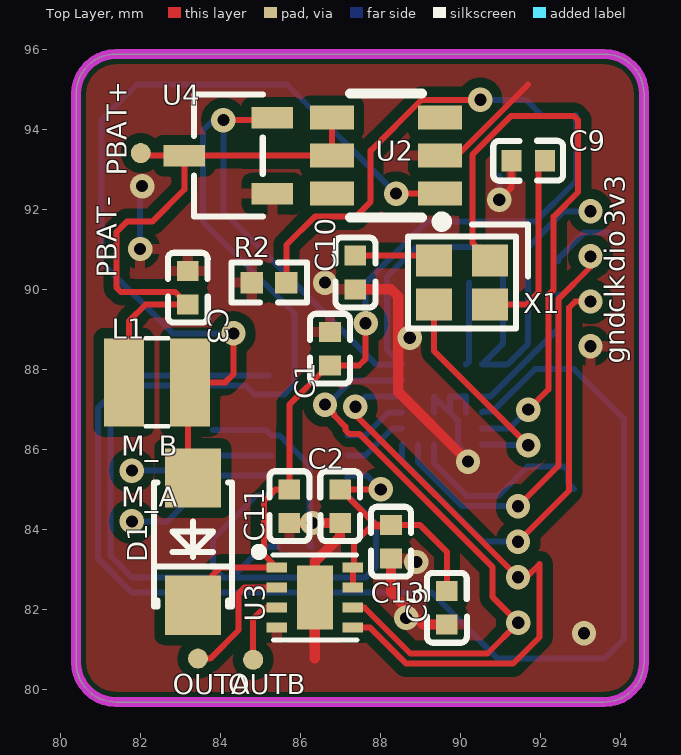
[diagram p0: Top Layer view]
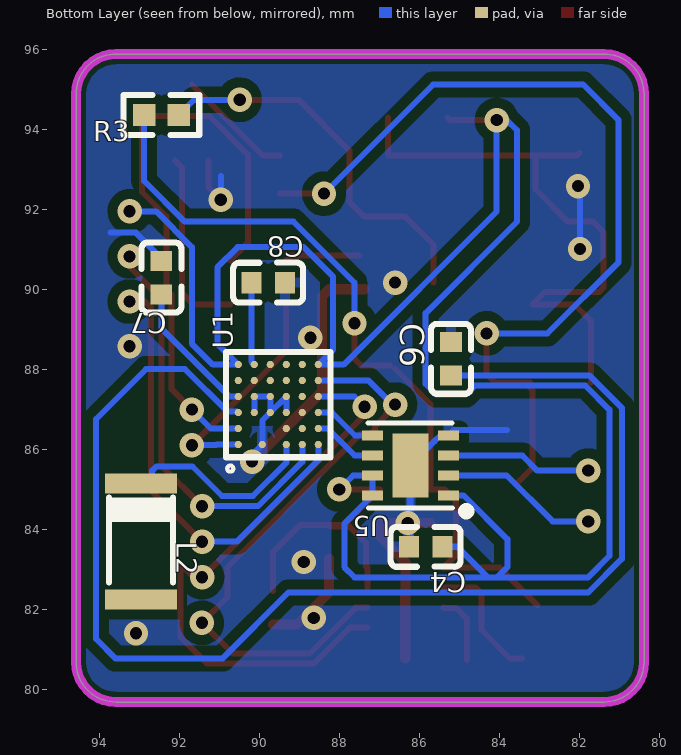
[diagram p1: Bottom Layer view, seen from below]
# Altium PCB MISC49870.pcbdoc
Units mm, origin at the board's own origin, x right, y up, seen from the top; angles counter-clockwise.
Board outline 14.2 x 16.2 mm, 2 copper layers (Top Layer, Bottom Layer), stack 1.58 mm thick; 33 components, 24 nets, 108 pads, 30 vias.

## Layer stack, top to bottom
Top Solder Mask Layer: solder mask 0.01, Dk 3.3
Top Layer: signal copper 0.035
Dielectric1: surface 1.51, FR4, Dk 4.5
Bottom Layer: signal copper 0.035
Bottom Solder Mask Layer: solder mask 0.01, Dk 3.3

## Board outline
81.391,95.885 ccw(c81.391,94.885) 80.391,94.885 80.391,80.685 ccw(c81.391,80.685) 81.391,79.685 93.591,79.685 ccw(c93.591,80.685) 94.591,80.685 94.591,94.885 ccw(c93.591,94.885) 93.591,95.885

## Design rules (kind name [scope] priority, off if disabled: settings)
BoardOutlineClearance copperThickness2oz_1 [All] p2 off: genericclearance=0.203 ignorepadtopadclearanceinfootprint=FALSE except(0: Arc-SplitContinuation Track-SplitContinuation SMDPad-SplitContinuation THPad-SplitContinuation Via-SplitContinuation Fill-SplitContinuation Region-SplitContinuation Poly-SplitContinuation Text-SplitContinuation Hole-SplitContinuation; 0.152: Arc-CutoutEdge SMDPad-CutoutEdge THPad-CutoutEdge Via-CutoutEdge Fill-CutoutEdge Region-CutoutEdge Text-CutoutEdge; 0.176: Hole-OutlineEdge Hole-CutoutEdge; 0.254: Poly-OutlineEdge Poly-CutoutEdge; 0.3: Arc-OutlineEdge Track-OutlineEdge SMDPad-OutlineEdge THPad-OutlineEdge Via-OutlineEdge Fill-OutlineEdge Region-OutlineEdge Text-OutlineEdge Track-CutoutEdge)
BoardOutlineClearance copperThickness1oz_1 [All] p4: genericclearance=0.102 ignorepadtopadclearanceinfootprint=FALSE except(0: Arc-SplitContinuation Track-SplitContinuation SMDPad-SplitContinuation THPad-SplitContinuation Via-SplitContinuation Fill-SplitContinuation Region-SplitContinuation Poly-SplitContinuation Text-SplitContinuation Hole-SplitContinuation; 0.152: SMDPad-CutoutEdge THPad-CutoutEdge Via-CutoutEdge Fill-CutoutEdge Region-CutoutEdge Text-CutoutEdge; 0.176: Hole-OutlineEdge Hole-CutoutEdge; 0.254: Poly-OutlineEdge Poly-CutoutEdge; 0.3: Arc-OutlineEdge Track-OutlineEdge SMDPad-OutlineEdge THPad-OutlineEdge Via-OutlineEdge Fill-OutlineEdge Region-OutlineEdge Text-OutlineEdge Arc-CutoutEdge Track-CutoutEdge)
Clearance copperThickness2oz [All] p1 off: gap=0.203 ignorepadtopadclearanceinfootprint=FALSE except(0.152: SMDPad-Track SMDPad-SMDPad THPad-Track SMDPad-THPad THPad-THPad Track-Via SMDPad-Via THPad-Via Via-Via Fill-Track Region-Track Fill-SMDPad Region-SMDPad Fill-THPad Region-THPad Fill-Via Region-Via Fill-Fill Fill-Region Region-Region Arc-Track Arc-SMDPad Arc-THPad Arc-Via Fill-Arc Region-Arc Arc-Arc Text-Track SMDPad-Text Text-THPad Text-Via Fill-Text Region-Text Arc-Text Text-Text; 0.176: Hole-Track Hole-SMDPad Hole-THPad Hole-Via Fill-Hole Region-Hole Hole-Arc Hole-Text; 0.254: Poly-Track Poly-SMDPad Poly-THPad Poly-Via Poly-Fill Poly-Region Poly-Poly Poly-Arc Poly-Text Poly-Hole)
Clearance copperThickness1oz [All] p3: gap=0.102 ignorepadtopadclearanceinfootprint=FALSE except(0.152: SMDPad-Track SMDPad-SMDPad THPad-Track SMDPad-THPad THPad-THPad Track-Via SMDPad-Via THPad-Via Via-Via Fill-Track Region-Track Fill-SMDPad Region-SMDPad Fill-THPad Region-THPad Fill-Via Region-Via Fill-Fill Fill-Region Region-Region Arc-Track Arc-SMDPad Arc-THPad Arc-Via Fill-Arc Region-Arc Arc-Arc Text-Track SMDPad-Text Text-THPad Text-Via Fill-Text Region-Text Arc-Text Text-Text; 0.176: Hole-Track Hole-SMDPad Hole-THPad Hole-Via Fill-Hole Region-Hole Hole-Arc Hole-Text; 0.254: Poly-Track Poly-SMDPad Poly-THPad Poly-Via Poly-Fill Poly-Region Poly-Poly Poly-Arc Poly-Text Poly-Hole)
DiffPairsRouting differentialPair [All] p1: maxlimit=0.152 minlimit=0.152 mostfreqgap=0.152 toplayer_minwidth=0.127 toplayer_prefwidth=0.254 toplayer_maxwidth=2.54 toplayer_mingap=0.152 toplayer_prefgap=0.152 toplayer_maxgap=0.152 bottomlayer_minwidth=0.127 bottomlayer_prefwidth=0.254 bottomlayer_maxwidth=2.54 bottomlayer_mingap=0.152 bottomlayer_prefgap=0.152 bottomlayer_maxgap=0.152 maxuncoupledlength=0.254
HoleToHoleClearance otherClearance [All] p1: gap=0.3 allowstackedmicrovias=TRUE
Length netLength [All] p1: minlimit=0 maxlimit=0
MatchedLengths netLengthTolerance [All] p1: tolerance=25.4
PasteMaskExpansion pasteMaskExpansion [All] p1: expansion=0
PlaneConnect innerPlane [All] p1: planeconnectstyle=Relief reliefexpansion=0.508 reliefentries=4 reliefconductorwidth=0.254 reliefairgap=0.254
PolygonConnect copperRegion [(InNet('GND'))] p1: connectstyle=Relief reliefconductorwidth=0.254 reliefentries=4 polygonreliefangle="90 Angle" airgapwidth=0.254 via.connectstyle=Relief via.reliefconductorwidth=0.254 via.reliefentries=4 via.polygonreliefangle="90 Angle" via.airgapwidth=0.254
RoutingVias viaSize [All] p1: holewidth=0.305 width=0.61 viastyle="Through Hole" minholewidth=0.3 minwidth=0.5 maxholewidth=6.3 maxwidth=10
SolderMaskExpansion solderMaskExpansion [IsVia] p1: expansion=-25.4 istentingtop=TRUE
SolderMaskExpansion solderMaskExpansion [All] p2: expansion=0.051 istentingtop=FALSE
Width copperThickness2oz_2 [All] p1 off: maxlimit=2.54 minlimit=0.203 preferedwidth=0.254
Width copperThickness1oz_2 [All] p2: maxlimit=2.54 minlimit=0.127 preferedwidth=0.254

## Components (designator, comment, footprint, x,y, rotation, side; value= is the part's Value field where it differs from the comment)
3v3 "" Test-Point-0.5mm 93.251,91.953 r0 top
C1 "100nF" C0402 86.741,88.519 r270 top
C2 "100nF" C0402 86.995,84.582 r90 top
C3 "10uF" C0402 83.185,90.043 r270 top
C4 "10uF" C0402 85.852,83.566 r0 bottom
C5 "100nF" C0402 89.662,82.042 r90 top
C6 "100nF" C0402 85.217,88.265 r270 bottom
C7 "100nF" C0402 92.456,90.297 r270 bottom
C8 "100nF" C0402 89.789,90.17 r0 bottom
C9 "12pF" C0402 91.694,93.218 r0 top
C10 "12pF" C0402 87.376,90.424 r90 top
C11 "100nF" C0402 85.725,84.582 r90 top
C13 "10uF" C0402 88.265,83.693 r270 top
clk "" Test-Point-0.5mm 93.251,89.698 r0 top
D1 "SS24L" SOD-123FL_L2.8-W1.8-LS3.7-R-RD 83.312,83.693 r90 top
dio "" Test-Point-0.5mm 93.251,90.825 r0 top
gnd "" Test-Point-0.5mm 93.251,88.582 r0 top
L1 "4.7uH" IND-SMD_L2.5-W2.0_VLS2520X 82.414,87.68 r180 top
L2 "KH-3216-H0209" ANT-SMD_L3.2-W1.6-KH-3216F245C04 92.964,83.693 r270 bottom
M_A "" Test-Point-0.5mm 81.771,84.192 r0 top
M_B "" Test-Point-0.5mm 81.771,85.462 r0 top
OUTA "" Test-Point-0.5mm 83.439,80.772 r0 top
OUTB "" Test-Point-0.5mm 84.819,80.741 r0 top
PBAT+ "" Test-Point-0.5mm 82.009,93.409 r0 top
PBAT- "" Test-Point-0.5mm 81.993,91.012 r0 top
R2 "9.1kΩ" R0402 85.217,90.17 r0 top
R3 "110kΩ" R0402 92.456,94.361 r0 bottom
U1 "NRF52810-CAAA-R" WLCSP-33_L2.5-W2.5-P0.40_NRF52810-CAAA-R 89.535,87.122 r90 bottom
U2 "MSY7208ABC" SOT-23-6_L2.9-W1.6-P0.95-LS2.8-BR 88.138,93.345 r0 top
U3 "DRV8837DSGR" WSON-8_L2.0-W2.0-P0.50-TL-EP 86.36,82.296 r0 top
U4 "XC6206P332MR" SOT-23-3_L3.0-W1.7-P0.95-LS2.9-BR 84.201,93.345 r0 top
U5 "DRV8837DSGR" WSON-8_L2.0-W2.0-P0.50-TL-EP 86.233,85.598 r0 bottom
X1 "32MHz" CRYSTAL-SMD_4P-L2.0-W1.6-BL 90.043,90.17 r180 top

## Footprints (in the part's own frame and the unit in brackets; to place one, negate y for a bottom-side part, rotate by r counter-clockwise, add the part's x,y. Pads: shape width x height; smd on the part's side, far side on the other; paste and mask are expansions set on the pad)
ANT-SMD_L3.2-W1.6-KH-3216F245C04 [mm]
  rect 0.5x1.8 smd: 1(-1.45,0) 2(1.45,0)
  silkscreen extent -1.1,-0.8 1.02,0.8
C0402 [mm]
  rect 0.5x0.54 smd: 1(-0.42,0) 2(0.42,0)
  silkscreen extent -0.87,-0.5 0.87,0.5
CRYSTAL-SMD_4P-L2.0-W1.6-BL [mm]
  rect 0.9x0.8 smd: 1(-0.7,-0.55) 2(0.7,-0.55) 3(0.7,0.55) 4(-0.7,0.55)
  silkscreen extent -1.65,-1.45 1.35,1.15
IND-SMD_L2.5-W2.0_VLS2520X [mm]
  rect 1x2.2 smd: 1(-0.83,0) 2(0.83,0)
  silkscreen extent -0.29,-1.1 0.29,1.1
R0402 [mm]
  rect 0.566x0.54 smd paste-100 mask+0.051: 1(-0.433,0) 2(0.433,0)
  silkscreen extent -0.94,-0.5 0.94,0.5
SOD-123FL_L2.8-W1.8-LS3.7-R-RD [mm]
  rect 1.48x1.4 smd paste+0 mask+0.05: 1(1.59,0) 2(-1.59,0)
  silkscreen extent -1.62,-0.98 1.48,0.98
SOT-23-3_L3.0-W1.7-P0.95-LS2.9-BR [mm]
  rect 1.037x0.532 smd: 1(1.101,-0.95) 2(1.101,0.95) 3(-1.101,0)
  silkscreen extent -0.86,-1.53 0.86,1.53
SOT-23-6_L2.9-W1.6-P0.95-LS2.8-BR [mm]
  rect 1.1x0.6 smd paste+0 mask+0.051: 1(1.35,-0.95) 2(1.35,0) 3(1.35,0.95) 4(-1.35,0.95) 5(-1.35,0) 6(-1.35,-0.95)
  silkscreen extent -0.9,-1.78 1.52,1.55
Test-Point-0.5mm [mm]
  round 0.5 smd: 1(0,0)
WLCSP-33_L2.5-W2.5-P0.40_NRF52810-CAAA-R [mm]
  round 0.182 smd paste-100 mask+0.051: A1(-1,1) A2(-0.6,1) A3(-0.2,1) A4(0.2,1) A5(0.6,1) A6(1,1) B3(-0.2,0.6) B4(0.2,0.6) B5(0.6,0.6) B6(1,0.6) C1(-1,0.4) D3(-0.2,0.2) D4(0.2,0.2) D5(0.6,0.2) D6(1,0.2) E1(-1,-0.2) E2(-0.6,-0.2) E3(-0.2,-0.2) E4(0.2,-0.2) E5(0.6,-0.2) E6(1,-0.2) F1(-1,-0.6) F2(-0.6,-0.6) F3(-0.2,-0.6) F4(0.2,-0.6) F5(0.6,-0.6) F6(1,-0.6) G1(-1,-1) G2(-0.6,-1) G3(-0.2,-1) G4(0.2,-1) G5(0.6,-1) G6(1,-1)
  silkscreen extent -1.68,-1.31 1.32,1.31
WSON-8_L2.0-W2.0-P0.50-TL-EP [mm]
  rect 0.521x0.25 smd paste+0 mask+0.05: 1(-0.95,0.75) 2(-0.95,0.25) 3(-0.95,-0.25) 4(-0.95,-0.75) 5(0.95,-0.75) 6(0.95,-0.25) 7(0.95,0.25) 8(0.95,0.75)
  rect 0.9x1.6 smd paste+0 mask+0.05: 9(0,0)
  silkscreen extent -1.47,-1.06 1.06,1.22

## Via types
v1: diameter 0.61, hole 0.305, Top Layer to Bottom Layer, 30 vias

## Nets (pads, with @x,y where several pads share a name; then routed paths per layer and width w, separated by ;. In a path a pad name is that pad's centre, name@x,y a point inside that pad or via, vN(x,y) a via of type N, cw(c..) or ccw(c..) an arc to the next point about the centre after c; other vN are vias at no path point)
3V3: 3v3.1 C2.2 C4.1 C5.2 C13.1 U1.A6 U1.G6 U3.7 U3.8 U4.2 U5.1 U5.7 U5.8 | length 62.8
  Top Layer w0.15: v1(84.074,94.234) 85.241,94.234 U4.2 ; U3.7 U3.8 87.341,83.077 87.341,83.658 87.757,84.074 88.226,84.074 C13.1 ; v1(88.011,85.002) C2.2 87.884,84.113 C13.1 ; C5.2 89.662,83.439 88.988,84.113 C13.1
  Bottom Layer w0.15: U5.1 84.902,84.848 83.811,83.756 83.811,83.058 84.065,82.804 ; v1(88.011,85.002) 87.665,85.348 U5.7 U5.8 87.884,84.147 87.884,83.058 87.63,82.804 84.297,82.804 84.065,82.804 ; v1(93.251,91.953) 92.588,91.953 91.694,91.059 91.694,88.646 91.17,88.122 U1.A6 91.059,88.646 91.059,90.551 90.551,91.059 88.9,91.059 88.162,90.321 88.162,88.495 U1.G6 87.9,88.122 84.074,91.948 v1(84.074,94.234) 83.82,94.234 83.566,93.98 83.566,91.694 85.852,89.408 85.852,87.639 85.581,87.368 84.853,87.368 84.628,87.593 81.853,87.593 81.256,86.996 81.256,83.336 81.788,82.804 84.065,82.804
  Bottom Layer w0.16: 84.297,82.804 85.059,83.566 C4.1
8V: C1.2 C11.2 D1.2 R3.2 U3.1 | length 19.5
  Top Layer w0.15: D1.2@83.058,82.103 84.001,83.046 U3.1 85.09,83.366 85.09,84.709 85.383,85.002 C11.2 85.725,87.122 C1.2@86.614,88.011 ; C1.2 87.464,88.099 87.63,88.265 v1(87.63,89.154)
  Bottom Layer w0.15: v1(87.63,89.154) 87.63,90.17 89.154,91.694 91.873,91.694 92.889,92.71 R3.2
$1N14: D1.1 L1.1 U2.1 | length 22.5
  Top Layer w0.15: L1.1 L1.1@83.371,87.68 ; D1.1@83.566,85.156 83.185,85.537 83.185,87.494 L1.1@83.371,87.68 ; v1(84.328,88.9) 84.328,87.884 84.124,87.68 L1.1@83.371,87.68 ; v1(88.392,92.395) U2.1
  Bottom Layer w0.15: v1(84.328,88.9) 82.804,88.9 81.026,90.678 81.026,94.234 81.915,95.123 85.664,95.123 v1(88.392,92.395)
$1N25: OUTA.1 U3.2 | length 3.2
  Top Layer w0.15: OUTA.1 83.742,80.772 84.455,81.485 84.455,82.4 84.605,82.55 85.406,82.55 U3.2
$1N26: OUTB.1 U3.3 | length 1.7
  Top Layer w0.15: OUTB.1 84.819,81.771 85.09,82.042 85.406,82.042 U3.3
$1N37: C6.2 U1.A3 | length 32.8
  Bottom Layer w0.15: C6.2 81.749,87.845 80.945,87.041 80.945,83.266 81.788,82.423 89.281,82.423 90.932,80.772 93.599,80.772 94.091,81.264 94.091,86.757 92.837,88.011 91.87,88.011 90.811,86.952 90.565,86.952 U1.A3
$1N38: C7.2 U1.A4 | length 3.5
  Bottom Layer w0.15: U1.A4 90.751,87.322 92.456,89.027 C7.2
$1N39: C8.2 U1.B6 | length 2.1
  Bottom Layer w0.15: U1.B6 90.209,88.196 C8.2
$1N43: U1.A1 X1.3 | length 5.7
  Top Layer w0.15: X1.3 89.343,88.457 v1(91.694,86.106)
  Bottom Layer w0.15: U1.A1 91.075,86.122 91.091,86.106 v1(91.694,86.106)
$1N44: U1.A2 X1.1 | length 15
  Top Layer w0.15: X1.1 90.297,91.166 90.297,93.37 91.267,94.34 92.837,94.34 92.943,94.234 92.943,92.435 92.329,91.821 92.329,89.994 92.204,89.869 92.204,88.013 92.202,88.011 92.202,87.503 v1(91.694,86.995)
  Bottom Layer w0.15: U1.A2 91.221,86.522 v1(91.694,86.995)
$1N46: C9.2 X1.4 | length 4.7
  Top Layer w0.15: X1.4 91.652,89.62 91.948,89.916 91.948,93.052 C9.2
$1N47: C10.2 X1.2 | length 1.9
  Top Layer w0.15: C10.2@87.503,90.844 89.219,90.844 X1.2
$1N49: L2.1 U1.E1 | length 5
  Bottom Layer w0.15: U1.E1 89.335,85.671 90.17,84.836 90.942,84.836 91.68,85.574 92.583,85.574 92.689,85.468 92.689,85.164 L2.1@92.837,85.016
$1N57: R2.2 R3.1 U2.3 | length 9.7
  Top Layer w0.15: R2.2 85.65,91.111 86.36,91.821 87.385,91.821 87.757,92.193 87.757,93.472 89.027,94.742 v1(90.499,94.742)
  Bottom Layer w0.15: v1(90.499,94.742) 91.642,94.742 R3.1
$1N60: M_B.1 U5.3 | length 3.7
  Bottom Layer w0.15: v1(81.788,85.471) 83.058,85.471 83.435,85.848 U5.3
$1N61: M_A.1 U5.2 | length 4
  Bottom Layer w0.15: v1(81.788,84.201) 82.677,84.201 83.824,85.348 U5.2
BAT+: C3.2 L1.2 PBAT+.1 U2.4 U2.5 U4.3 | length 15.3
  Top Layer w0.15: L1.2@81.711,87.68 81.711,89.204 82.13,89.623 C3.2 82.871,89.937 81.513,89.937 81.407,90.043 81.407,91.44 81.661,91.694 82.296,91.694 83.1,92.498 U4.3 ; PBAT+.1 82.072,93.345 U4.3 ; U2.4 U2.5 U4.3
DIR1: U1.G3 U5.5 | length 1.6
  Bottom Layer w0.15: U5.5 87.618,86.348 88.192,86.922 U1.G3
DIR2: U1.G2 U5.6 | length 1.6
  Bottom Layer w0.15: U5.6 87.626,85.848 88.3,86.522 U1.G2
GND: C1.1 C2.1 C3.1 C4.2 C5.1 C6.1 C7.1 C8.1 C9.1 C10.1 C11.1 C13.2 gnd.1 PBAT-.1 R2.1 U1.B3 U1.B4 U1.C1 U1.D3 U1.D4 U1.E3 U1.E4 U2.2 U3.4 U3.9 U4.1 U5.4 U5.9 | length 29.7
  Top Layer w0.15: U2.2 89.916,93.345 91.694,95.123 ; v1(90.973,92.243) 91.274,92.544 C9.1
  Top Layer w0.25: C11.1 v1(86.299,84.162) C2.1 86.995,83.82 86.36,83.185 U3.9 ; C13.2 88.265,82.423 89.066,81.622 C5.1
  Top Layer w0.254: 86.36,80.772 U3.9 ; C10.1 88.265,90.004 88.445,89.824 88.445,87.442 v1(90.189,85.697)
  Bottom Layer w0.15: v1(81.993,91.012) 81.993,92.534 v1(82.042,92.583) ; 83.82,86.487 85.144,86.487 U5.4 85.483,86.348 85.631,86.2 85.638,86.2 85.771,86.067 85.771,86.06 U5.9 ; U1.E3 U1.E4 ; U1.E4 U1.D3 ; U1.B3 U1.B4 U1.D4 U1.D3 ; v1(90.189,85.697) 90.189,85.867 U1.C1 89.935,86.722 U1.D3 ; v1(90.973,92.243) 90.973,92.837 ; C7.1 92.456,90.782 93.095,91.421 93.726,91.421
  Bottom Layer w0.16: U5.9 86.233,83.605 C4.2
  other v1: 93.091,81.407 88.646,81.788 88.9,83.185 93.251,88.582 88.733,88.792 86.614,90.17
PWM1: U1.G4 U3.5 | length 15
  Top Layer w0.15: U3.5 87.745,81.546 88.644,80.647 91.315,80.647 91.977,81.309 91.977,83.132 91.649,82.804 v1(91.44,82.804) 87.376,86.868 v1(87.376,87.068)
  Bottom Layer w0.15: v1(87.376,87.068) 87.63,87.322 U1.G4
PWM2: U1.G5 U3.6 | length 14.7
  Top Layer w0.15: v1(86.614,87.122) 86.844,86.892 86.844,86.848 87.122,86.57 87.122,86.487 87.228,86.381 87.482,86.381 90.805,83.058 90.805,82.306 v1(91.445,81.666) 90.678,80.899 88.748,80.899 87.601,82.046 U3.6
  Bottom Layer w0.15: v1(86.614,87.122) 86.678,87.122 87.283,87.727 88.53,87.727 U1.G5
SWDCLK: clk.1 U1.G1 | length 11.1
  Top Layer w0.15: v1(91.44,83.693) 92.719,84.972 92.719,89.548 92.869,89.698 v1(93.251,89.698)
  Bottom Layer w0.15: U1.G1 88.535,85.733 90.576,83.693 v1(91.44,83.693)
SWDIO: dio.1 U1.F1 | length 10.4
  Top Layer w0.15: v1(91.44,84.582) 92.456,85.598 92.456,89.764 93.251,90.56 v1(93.251,90.825)
  Bottom Layer w0.15: U1.F1 88.935,85.69 90.043,84.582 v1(91.44,84.582)
pads on no net: L2.2 U1.A5 U1.B5 U1.D5 U1.D6 U1.E2 U1.E5 U1.E6 U1.F2 U1.F3 U1.F4 U1.F5 U1.F6 U2.6

## Polygon pours and split planes (outlines as drawn)
GND on Top Layer (solid, remove dead copper, pour order 2): 76.2,97.663 76.2,76.2 99.06,76.2 99.06,97.663
GND on Bottom Layer (solid, remove dead copper, pour order 4): 76.708,97.028 76.708,76.454 97.663,76.454 97.663,97.028
GND on Top Layer (solid, remove dead copper, pour order 0): 79.375,96.012 79.375,86.487 92.202,86.487 92.202,96.012

## Keep-outs
Board Outline Layer:
  the board outline again, w0.254